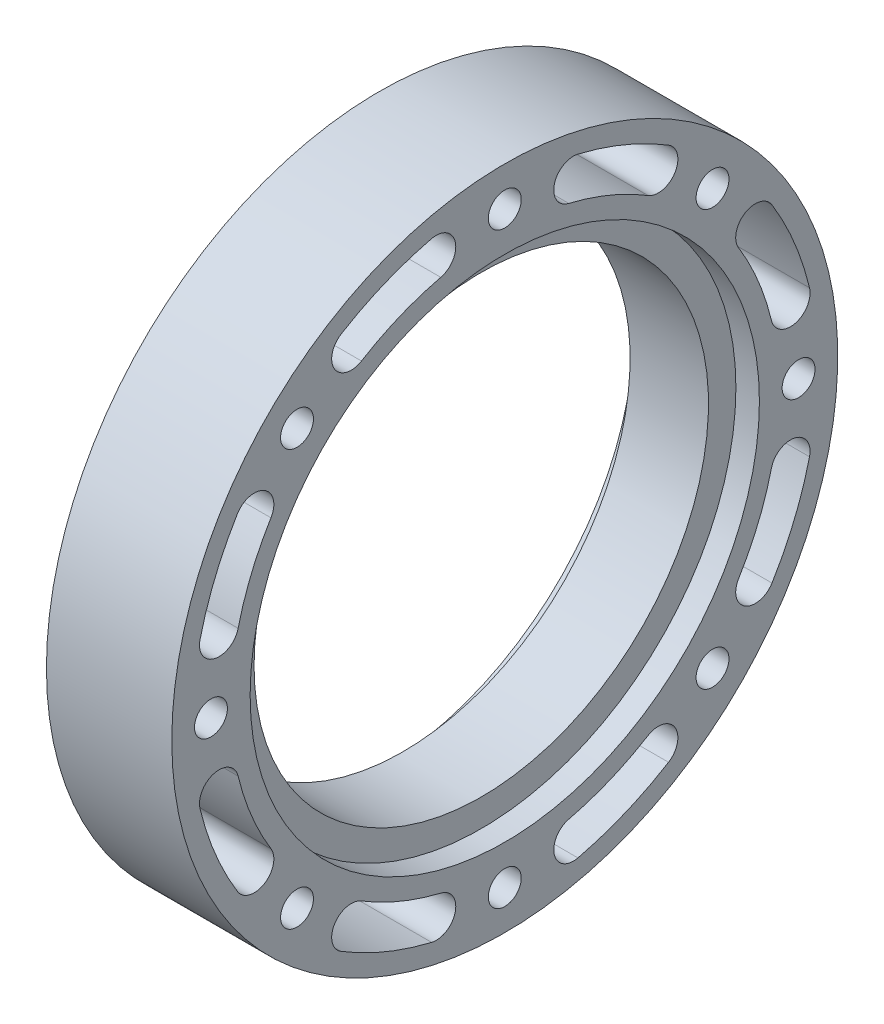
SolidWorks part; units mm, degrees
material "ABS"
ref_plane "前视基准面" through (0, 0, 0) normal (0, 0, 1) x (1, 0, 0)
ref_plane "上视基准面" through (0, 0, 0) normal (0, 1, 0) x (1, 0, 0)
ref_plane "右视基准面" through (0, 0, 0) normal (1, 0, 0) x (0, 0, -1)
other "Configuration Table"
sketch "草图1" plane through (0, 0, 0) normal (0, 1, 0) x (1, 0, 0)
  line L0 (-880.6263, 0) -> (43150.6864, 0) construction
  line L1 (-5, 29) -> (-5, 32.5)
  line L2 (-5, 32.5) -> (-8, 32.5)
  line L3 (-8, 32.5) -> (-8, 42.5)
  line L4 (-8, 42.5) -> (8, 42.5)
  line L5 (8, 42.5) -> (8, 32.5)
  line L6 (8, 32.5) -> (5, 32.5)
  line L7 (5, 32.5) -> (5, 29)
  line L8 (5, 29) -> (-5, 29)
  point P11 (0, 29)
  dimension "D1" = 58
  dimension "D2" = 10
  dimension "D3" = 16
  dimension "D4" = 65
  dimension "D5" = 85
revolve "旋转1" add sketch "草图1" angle 360 about L0
sketch "草图2" plane through (8, 0, 0) normal (1, 0, 0) x (0, 0, -1)
  line L0 (8.7542, 36.4639) -> (0, 0) construction
  line L1 (0, 0) -> (19.5937, 31.974) construction
  line L2 (0, 37.5) -> (0, 0) construction
  line L3 (14.3506, 34.6455) -> (0, 0) construction
  circle A0 centre (0, 0) radius 37.5 construction
  circle A1 centre (0, 37.5) radius 2.1
  circle A2 centre (26.5165, 26.5165) radius 2.1
  circle A3 centre (37.5, 0) radius 2.1
  circle A4 centre (26.5165, -26.5165) radius 2.1
  circle A5 centre (0, -37.5) radius 2.1
  circle A6 centre (-26.5165, -26.5165) radius 2.1
  circle A7 centre (-37.5, 0) radius 2.1
  circle A8 centre (-26.5165, 26.5165) radius 2.1
  arc A9 (8.7542, 36.4639) -> (19.5937, 31.974) centre (0, 0) cw construction
  arc A10 (20.8999, 34.1056) -> (9.3378, 38.8948) centre (0, 0) ccw
  arc A11 (18.2874, 29.8424) -> (8.1706, 34.0329) centre (0, 0) ccw
  arc A12 (18.2874, 29.8424) -> (20.8999, 34.1056) centre (19.5937, 31.974) ccw
  arc A13 (9.3378, 38.8948) -> (8.1706, 34.0329) centre (8.7542, 36.4639) ccw
  arc A14 (31.974, 19.5937) -> (36.4639, 8.7542) centre (0, 0) cw construction
  arc A15 (38.8948, 9.3378) -> (34.1056, 20.8999) centre (0, 0) ccw
  arc A16 (34.0329, 8.1706) -> (29.8424, 18.2874) centre (0, 0) ccw
  arc A17 (34.0329, 8.1706) -> (38.8948, 9.3378) centre (36.4639, 8.7542) ccw
  arc A18 (34.1056, 20.8999) -> (29.8424, 18.2874) centre (31.974, 19.5937) ccw
  arc A19 (36.4639, -8.7542) -> (31.974, -19.5937) centre (0, 0) cw construction
  arc A20 (34.1056, -20.8999) -> (38.8948, -9.3378) centre (0, 0) ccw
  arc A21 (29.8424, -18.2874) -> (34.0329, -8.1706) centre (0, 0) ccw
  arc A22 (29.8424, -18.2874) -> (34.1056, -20.8999) centre (31.974, -19.5937) ccw
  arc A23 (38.8948, -9.3378) -> (34.0329, -8.1706) centre (36.4639, -8.7542) ccw
  arc A24 (19.5937, -31.974) -> (8.7542, -36.4639) centre (0, 0) cw construction
  arc A25 (9.3378, -38.8948) -> (20.8999, -34.1056) centre (0, 0) ccw
  arc A26 (8.1706, -34.0329) -> (18.2874, -29.8424) centre (0, 0) ccw
  arc A27 (8.1706, -34.0329) -> (9.3378, -38.8948) centre (8.7542, -36.4639) ccw
  arc A28 (20.8999, -34.1056) -> (18.2874, -29.8424) centre (19.5937, -31.974) ccw
  arc A29 (-8.7542, -36.4639) -> (-19.5937, -31.974) centre (0, 0) cw construction
  arc A30 (-20.8999, -34.1056) -> (-9.3378, -38.8948) centre (0, 0) ccw
  arc A31 (-18.2874, -29.8424) -> (-8.1706, -34.0329) centre (0, 0) ccw
  arc A32 (-18.2874, -29.8424) -> (-20.8999, -34.1056) centre (-19.5937, -31.974) ccw
  arc A33 (-9.3378, -38.8948) -> (-8.1706, -34.0329) centre (-8.7542, -36.4639) ccw
  arc A34 (-31.974, -19.5937) -> (-36.4639, -8.7542) centre (0, 0) cw construction
  arc A35 (-38.8948, -9.3378) -> (-34.1056, -20.8999) centre (0, 0) ccw
  arc A36 (-34.0329, -8.1706) -> (-29.8424, -18.2874) centre (0, 0) ccw
  arc A37 (-34.0329, -8.1706) -> (-38.8948, -9.3378) centre (-36.4639, -8.7542) ccw
  arc A38 (-34.1056, -20.8999) -> (-29.8424, -18.2874) centre (-31.974, -19.5937) ccw
  arc A39 (-36.4639, 8.7542) -> (-31.974, 19.5937) centre (0, 0) cw construction
  arc A40 (-34.1056, 20.8999) -> (-38.8948, 9.3378) centre (0, 0) ccw
  arc A41 (-29.8424, 18.2874) -> (-34.0329, 8.1706) centre (0, 0) ccw
  arc A42 (-29.8424, 18.2874) -> (-34.1056, 20.8999) centre (-31.974, 19.5937) ccw
  arc A43 (-38.8948, 9.3378) -> (-34.0329, 8.1706) centre (-36.4639, 8.7542) ccw
  arc A44 (-19.5937, 31.974) -> (-8.7542, 36.4639) centre (0, 0) cw construction
  arc A45 (-9.3378, 38.8948) -> (-20.8999, 34.1056) centre (0, 0) ccw
  arc A46 (-8.1706, 34.0329) -> (-18.2874, 29.8424) centre (0, 0) ccw
  arc A47 (-8.1706, 34.0329) -> (-9.3378, 38.8948) centre (-8.7542, 36.4639) ccw
  arc A48 (-20.8999, 34.1056) -> (-18.2874, 29.8424) centre (-19.5937, 31.974) ccw
  point P21 (14.3506, 34.6455)
  point P34 (34.6455, 14.3506)
  point P41 (34.6455, -14.3506)
  point P48 (14.3506, -34.6455)
  point P55 (-14.3506, -34.6455)
  point P62 (-34.6455, -14.3506)
  point P69 (-34.6455, 14.3506)
  point P76 (-14.3506, 34.6455)
  point P81 (0, 0)
  dimension "D1" = 75
  dimension "D2" = 4.2
  dimension "D4" = 5
  dimension "D5" = 18
  dimension "D6" = 22.5
  dimension "D3" = 8
  dimension "D7" = 8
extrude "切除-拉伸1" cut sketch "草图2" against normal through all
